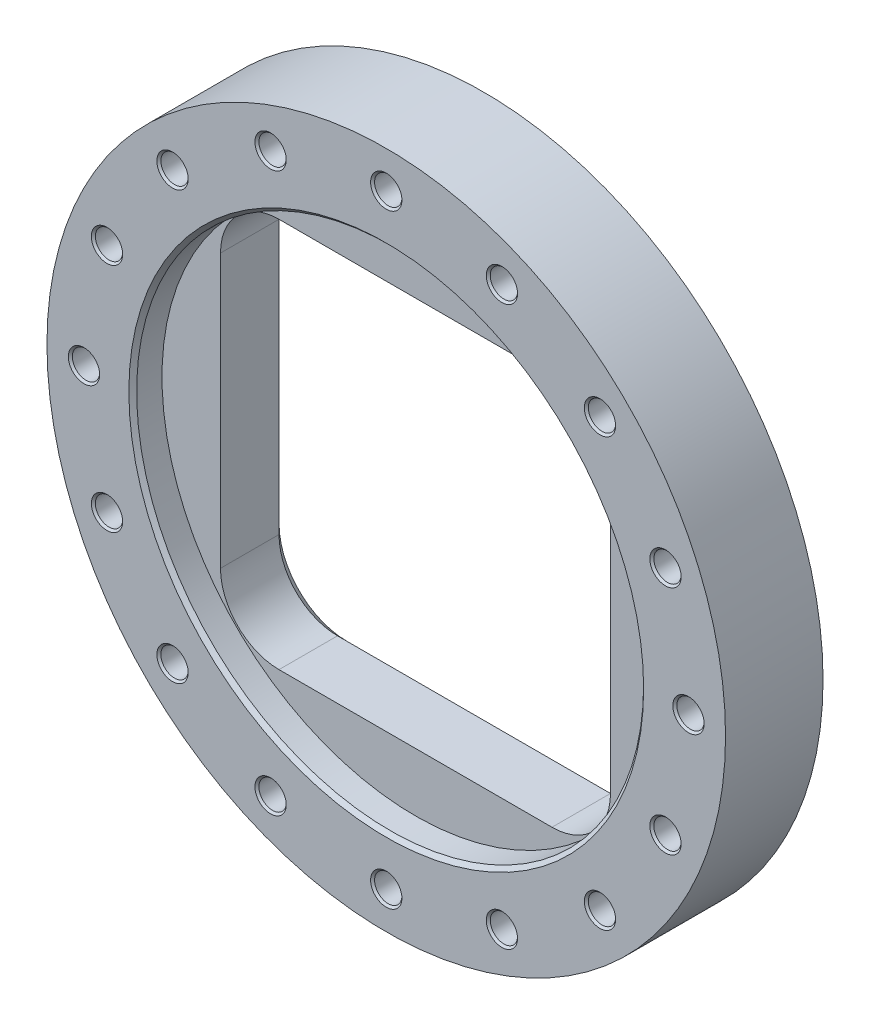
from build123d import *

# Parameters (mm, degrees)
SKETCH_1_R                    = 174
EXTRUDE_1_DEPTH               = 50
CUT_EXTRUDE_1_DEPTH           = 252.101573074
HOLE_WIZARD_M16_1_D           = 14
HOLE_WIZARD_M16_1_CSINK_D     = 16.05
HOLE_WIZARD_M16_1_CSINK_ANGLE = 90
PATTERN_CIRCULAR_1_COUNT      = 16
SKETCH_5_R                    = 130
CUT_EXTRUDE_2_DEPTH           = 15
CHAMFER_1_SIZE                = 2
CHAMFER_2_SIZE                = 5


with BuildPart() as part:
    # 草图1 → 凸台-拉伸1 (new body)
    with BuildSketch(Plane.XY):
        Circle(SKETCH_1_R)
    extrude(amount=EXTRUDE_1_DEPTH)

    # 草图2 → 切除-拉伸1 (cut, through all)
    with BuildSketch(Plane.XY.offset(50)):
        with BuildLine():
            Line((-70, 100), (70, 100))
            ThreePointArc((70, 100), (91.213203436, 91.213203436), (100, 70))
            Line((100, 70), (100, -70))
            ThreePointArc((100, -70), (91.213203436, -91.213203436), (70, -100))
            Line((70, -100), (-70, -100))
            ThreePointArc((-70, -100), (-91.213203436, -91.213203436), (-100, -70))
            Line((-100, -70), (-100, 70))
            ThreePointArc((-100, 70), (-91.213203436, 91.213203436), (-70, 100))
        make_face()
    extrude(amount=-CUT_EXTRUDE_1_DEPTH, mode=Mode.SUBTRACT)

    # M16 螺纹孔1 (through all)
    with Locations(Plane(origin=(0, 155, 50), x_dir=(1, 0, 0), z_dir=(0, 0, 1))):
        with Locations((0, 0)):
            hole_wizard_m16_1 = CounterSinkHole(HOLE_WIZARD_M16_1_D / 2, HOLE_WIZARD_M16_1_CSINK_D / 2, counter_sink_angle=HOLE_WIZARD_M16_1_CSINK_ANGLE)

    # 阵列(圆周)1: M16 螺纹孔1 ×16 about axis
    pattern_circular_1_axis = Axis((0, 0, 0), (0, 0, 1))
    for i in range(1, PATTERN_CIRCULAR_1_COUNT):
        add(hole_wizard_m16_1.rotate(pattern_circular_1_axis, i * 360 / PATTERN_CIRCULAR_1_COUNT), mode=Mode.SUBTRACT)

    # 草图5 → 切除-拉伸2 (cut)
    with BuildSketch(Plane.XY.offset(50)):
        Circle(SKETCH_5_R)
    extrude(amount=-CUT_EXTRUDE_2_DEPTH, mode=Mode.SUBTRACT)

    # 倒角1
    chamfer_1_edges = [part.edges().sort_by_distance(p)[0] for p in [
        (-130, 0, 50),
    ]]
    chamfer(chamfer_1_edges, length=CHAMFER_1_SIZE)

    # 倒角2
    chamfer_2_edges = [part.edges().sort_by_distance(p)[0] for p in [
        (-91.213203436, -91.213203436, 0),
        (-100, 0, 0),
        (-91.213203436, 91.213203436, 0),
        (0, 100, 0),
        (91.213203436, 91.213203436, 0),
        (100, 0, 0),
        (91.213203436, -91.213203436, 0),
        (0, -100, 0),
    ]]
    chamfer(chamfer_2_edges, length=CHAMFER_2_SIZE)


solid = part.part
